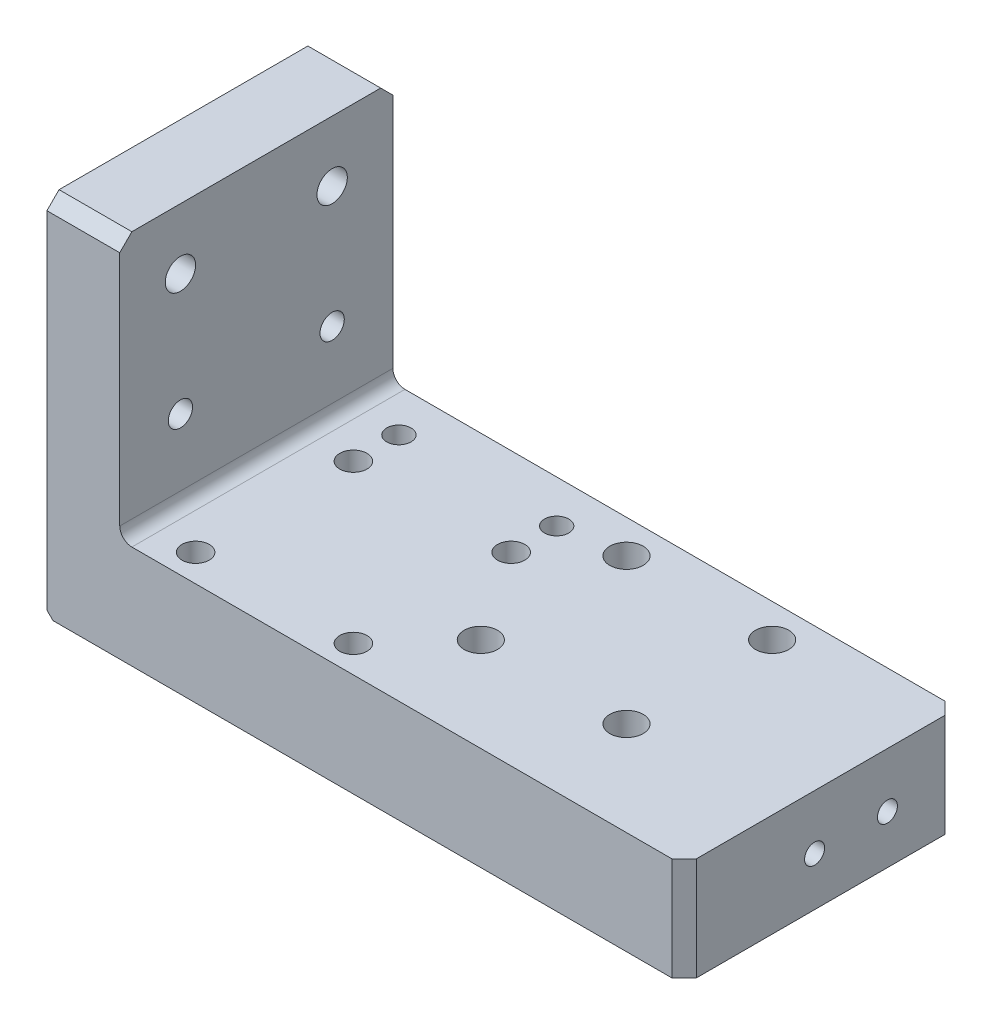
SolidWorks part; units mm, degrees
material "SS41"
ref_plane "Front Plane" through (0, 0, 0) normal (0, 0, 1) x (1, 0, 0)
ref_plane "Top Plane" through (0, 0, 0) normal (0, 1, 0) x (1, 0, 0)
ref_plane "Right Plane" through (0, 0, 0) normal (1, 0, 0) x (0, 0, -1)
sketch "Sketch1" plane through (0, 0, 0) normal (0, 0, 1) x (1, 0, 0)
  line L0 (0, 0) -> (0, 60)
  line L1 (0, 60) -> (12, 60)
  line L2 (12, 60) -> (12, 17)
  line L3 (12, 17) -> (105, 17)
  line L4 (105, 17) -> (105, 0)
  line L5 (105, 0) -> (0, 0)
  dimension "D1" = 17
  dimension "D2" = 60
  dimension "D3" = 12
  dimension "D4" = 105
extrude "Boss-Extrude1" add sketch "Sketch1" along normal mid plane 45
hole_wizard "Hole size per socket head cap screw type 1" positions "Sketch3" profile "Sketch2" counterbore size "M5" standard "Gb" end condition through all
sketch "Sketch3" plane through (0, 0, 0) normal (0, -1, 0) x (-1, 0, 0)
  line L0 (0, -22.5) -> (0, 22.5) construction
  line L1 (0, -22.5) -> (-105, -22.5) construction
  point P0 (-80, -7)
  point P2 (-56, -7)
  point P4 (-56, 17)
  point P6 (-80, 17)
  dimension "D1" = 24
  dimension "D2" = 24
  dimension "D3" = 15.5
  dimension "D4" = 56
sketch "Sketch2" plane through (80, 0, 7) normal (1, 0, 0) x (0, 0, -1)
  line L0 (0, 0) -> (0, 60)
  line L1 (0, 60) -> (2.75, 60)
  line L3 (2.75, 60) -> (2.75, 5.7)
  line L4 (2.75, 5.7) -> (5, 5.7)
  line L5 (5, 5.7) -> (5, 0)
  line L7 (5, 0) -> (0, 0)
  line L11 (0, -6.35) -> (0, 107.95) construction
  dimension "通孔孔直径" = 5.5
  dimension "通孔孔深度" = 60
  dimension "柱形沉头孔直径" = 10
  dimension "柱形沉头孔深度" = 5.7
hole_wizard "Ø4.5 (4.5) Diameter Hole1" positions "Sketch5" profile "Sketch4" hole size "Ø4.5" standard "Gb" end condition through all
sketch "Sketch5" plane through (0, 17, 0) normal (0, 1, 0) x (1, 0, 0)
  line L0 (0, -22.5) -> (0, 22.5) construction
  line L1 (0, -22.5) -> (105, -22.5) construction
  point P0 (20, 8)
  point P2 (46, 8)
  point P4 (20, -18)
  point P6 (46, -18)
  dimension "D1" = 26
  dimension "D2" = 26
  dimension "D3" = 4.5
  dimension "D4" = 20
sketch "Sketch4" plane through (20, 17, -8) normal (1, 0, 0) x (0, 0, 1)
  line L0 (0, 0) -> (0, 17)
  line L1 (0, 17) -> (2.25, 17)
  line L2 (2.25, 17) -> (2.25, 0)
  line L5 (2.25, 0) -> (0, 0)
  line L11 (0, -6.35) -> (0, 107.95) construction
  dimension "通孔孔直径" = 4.5
  dimension "通孔孔深度" = 17
hole_wizard "M4 Tapped Hole1" positions "Sketch7" profile "Sketch6" tap size "M4" standard "Gb"
sketch "Sketch7" plane through (105, 0, 0) normal (1, 0, 0) x (0, 0, -1)
  line L0 (-1, 8) -> (11, 8) construction
  line L5 (-22.5, 0) -> (22.5, 0) construction
  line L6 (-22.5, 0) -> (-22.5, 17) construction
  point P0 (-1, 8)
  point P2 (11, 8)
  dimension "D1" = 12
  dimension "D2" = 8
  dimension "D3" = 21.5
sketch "Sketch6" plane through (105, 8, 1) normal (0, 1, 0) x (0, 0, -1)
  line L0 (0, 0) -> (0, 11.0914)
  line L1 (0, 11.0914) -> (1.65, 10.1)
  line L2 (1.65, 10.1) -> (1.65, 0)
  line L5 (1.65, 0) -> (0, 0)
  line L10 (0, 11.0914) -> (-1.65, 10.1) construction
  line L11 (0, -6.35) -> (0, 107.95) construction
  dimension "螺纹孔钻头直径" = 3.3
  dimension "螺纹孔钻头深度" = 10.1
  dimension "导头角度" = 118
cosmetic thread "Cosmetic thread 1" parameters "D1"=8, "D2"=4
cosmetic thread "Cosmetic thread 2" parameters "D1"=8, "D2"=4
hole_wizard "M6 Tapped Hole1" positions "Sketch9" profile "Sketch8" tap size "M6" standard "Gb"
sketch "Sketch9" plane through (0, 0, 0) normal (-1, 0, 0) x (0, 0, 1)
  line L0 (22.5, 0) -> (-22.5, 0) construction
  point P0 (-12.5, 50)
  point P2 (12.5, 50)
  point P4 (-12.5, 10)
  point P6 (12.5, 10)
  dimension "D1" = 25
  dimension "D2" = 12.5
  dimension "D3" = 10
  dimension "D4" = 40
sketch "Sketch8" plane through (0, 50, -12.5) normal (0, 1, 0) x (0, 0, 1)
  line L0 (0, 0) -> (0, 16.5022)
  line L1 (0, 16.5022) -> (2.5, 15)
  line L2 (2.5, 15) -> (2.5, 0)
  line L5 (2.5, 0) -> (0, 0)
  line L10 (0, 16.5022) -> (-2.5, 15) construction
  line L11 (0, -6.35) -> (0, 107.95) construction
  dimension "螺纹孔钻头直径" = 5
  dimension "螺纹孔钻头深度" = 15
  dimension "导头角度" = 118
cosmetic thread "Cosmetic thread 3" parameters "D1"=12, "D2"=6
cosmetic thread "Cosmetic thread 4" parameters "D1"=12, "D2"=6
cosmetic thread "Cosmetic thread 5" parameters "D1"=12, "D2"=6
cosmetic thread "Cosmetic thread 6" parameters "D1"=12, "D2"=6
hole_wizard "Ø4.0 (4) Diameter Hole1" positions "Sketch11" profile "Sketch10" hole size "Ø4.0" standard "Gb"
sketch "Sketch11" plane through (0, 0, 0) normal (-1, 0, 0) x (0, 0, 1)
  line L0 (12.5, 10) -> (12.5, 50) construction
  line L3 (-12.5, 50) -> (-12.5, 10) construction
  point P0 (-12.5, 30)
  point P2 (12.5, 30)
sketch "Sketch10" plane through (0, 30, -12.5) normal (0, 1, 0) x (0, 0, 1)
  line L0 (0, 0) -> (0, 16.2017)
  line L1 (0, 16.2017) -> (2, 15)
  line L2 (2, 15) -> (2, 0)
  line L5 (2, 0) -> (0, 0)
  line L10 (0, 16.2017) -> (-2, 15) construction
  line L11 (0, -6.35) -> (0, 107.95) construction
  dimension "孔直径" = 4
  dimension "孔深度" = 15
  dimension "导头角度" = 118
hole_wizard "Ø4.0 (4) Diameter Hole2" positions "Sketch13" profile "Sketch12" hole size "Ø4.0" standard "Gb"
sketch "Sketch13" plane through (0, 0, 0) normal (0, -1, 0) x (-1, 0, 0)
  line L0 (-20, 15.5) -> (-20, 8) construction
  line L4 (-46, 15.5) -> (-46, 8) construction
  point P0 (-20, 15.5)
  point P2 (-46, 15.5)
  dimension "D1" = 7.5
sketch "Sketch12" plane through (20, 0, -15.5) normal (1, 0, 0) x (0, 0, -1)
  line L0 (0, 0) -> (0, 18.2017)
  line L1 (0, 18.2017) -> (2, 17)
  line L2 (2, 17) -> (2, 0)
  line L5 (2, 0) -> (0, 0)
  line L10 (0, 18.2017) -> (-2, 17) construction
  line L11 (0, -6.35) -> (0, 107.95) construction
  dimension "孔直径" = 4
  dimension "孔深度" = 17
  dimension "导头角度" = 118
chamfer "Chamfer1" distance 2 angle 45 4 edges at (105, 8.5, -22.5) (105, 8.5, 22.5) (6, 60, -22.5) (6, 60, 22.5)
chamfer "Chamfer2" distance 1 angle 45 1 edges at (0, 0, 0)
fillet "Fillet1" radius 2 1 edges at (12, 17, 0)
